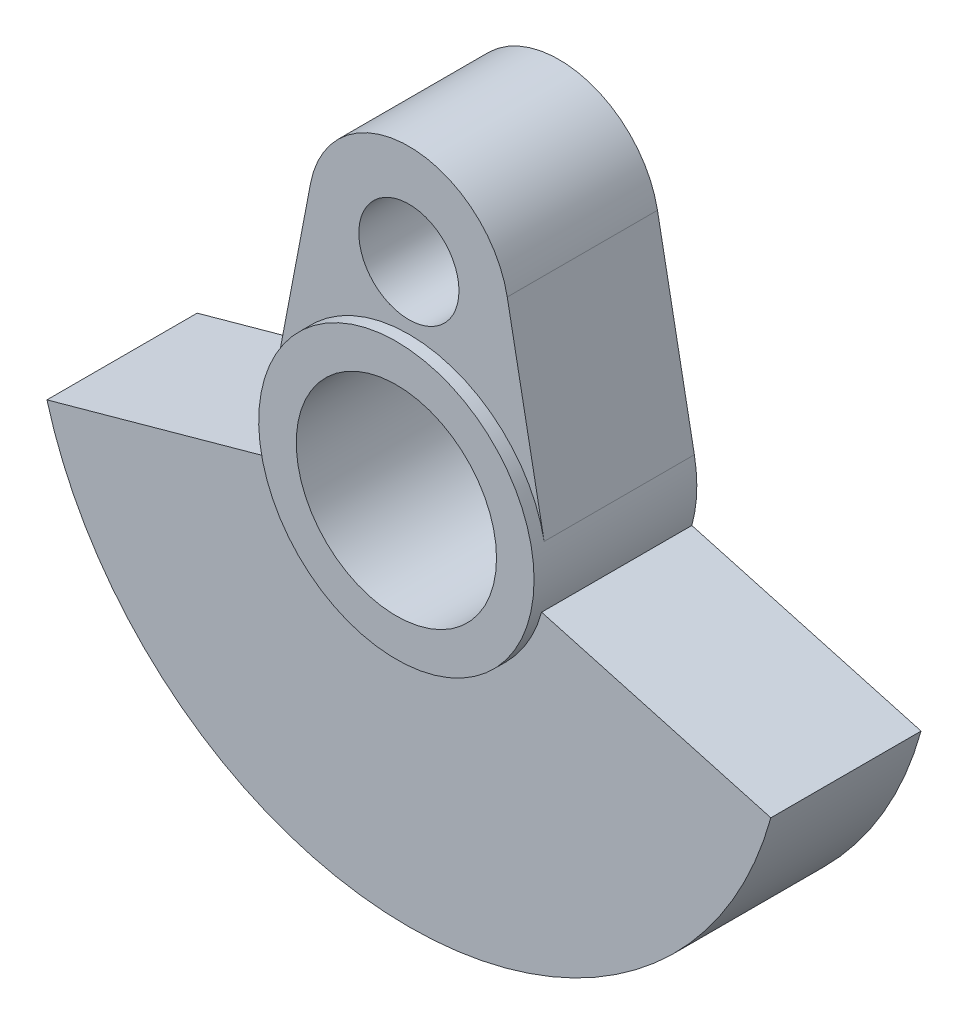
from build123d import *

# Parameters (mm, degrees)
SKETCH1_R           = 4
BOSS_EXTRUDE2_DEPTH = 6
SKETCH3_R           = 2
BOSS_EXTRUDE3_DEPTH = 6
SKETCH4_R           = 5.5
SKETCH4_R_2         = 4
BOSS_EXTRUDE4_DEPTH = 0.5


with BuildPart() as part:
    # Sketch1 → Boss-Extrude2 (new body)
    with BuildSketch(Plane.XY):
        with BuildLine():
            Line((-5.300838508, -1.466666667), (-14.456832295, -4))
            ThreePointArc((-14.456832295, -4), (0, -15), (14.456832295, -4))
            Line((14.456832295, -4), (5.300838508, -1.466666667))
            ThreePointArc((5.300838508, -1.466666667), (0, 5.5), (-5.300838508, -1.466666667))
        make_face()
        Circle(SKETCH1_R, mode=Mode.SUBTRACT)
    extrude(amount=BOSS_EXTRUDE2_DEPTH)

    # Sketch3 → Boss-Extrude3 (add)
    with BuildSketch(Plane.XY):
        with BuildLine():
            Line((-3.929058411, 8.75), (-5.402455316, 1.03125))
            ThreePointArc((-5.402455316, 1.03125), (0, 5.5), (5.402455316, 1.03125))
            Line((5.402455316, 1.03125), (3.929058411, 8.75))
            ThreePointArc((3.929058411, 8.75), (0, 12), (-3.929058411, 8.75))
        make_face()
        with Locations((0, 8)):
            Circle(SKETCH3_R, mode=Mode.SUBTRACT)
    extrude(amount=BOSS_EXTRUDE3_DEPTH)

    # Sketch4 → Boss-Extrude4 (add)
    with BuildSketch(Plane.XY.offset(6)):
        with Locations(Location((0, 0, 0), (0, 0, 169.193077125))):
            Circle(SKETCH4_R)
        Circle(SKETCH4_R_2, mode=Mode.SUBTRACT)
    extrude(amount=BOSS_EXTRUDE4_DEPTH)


solid = part.part
